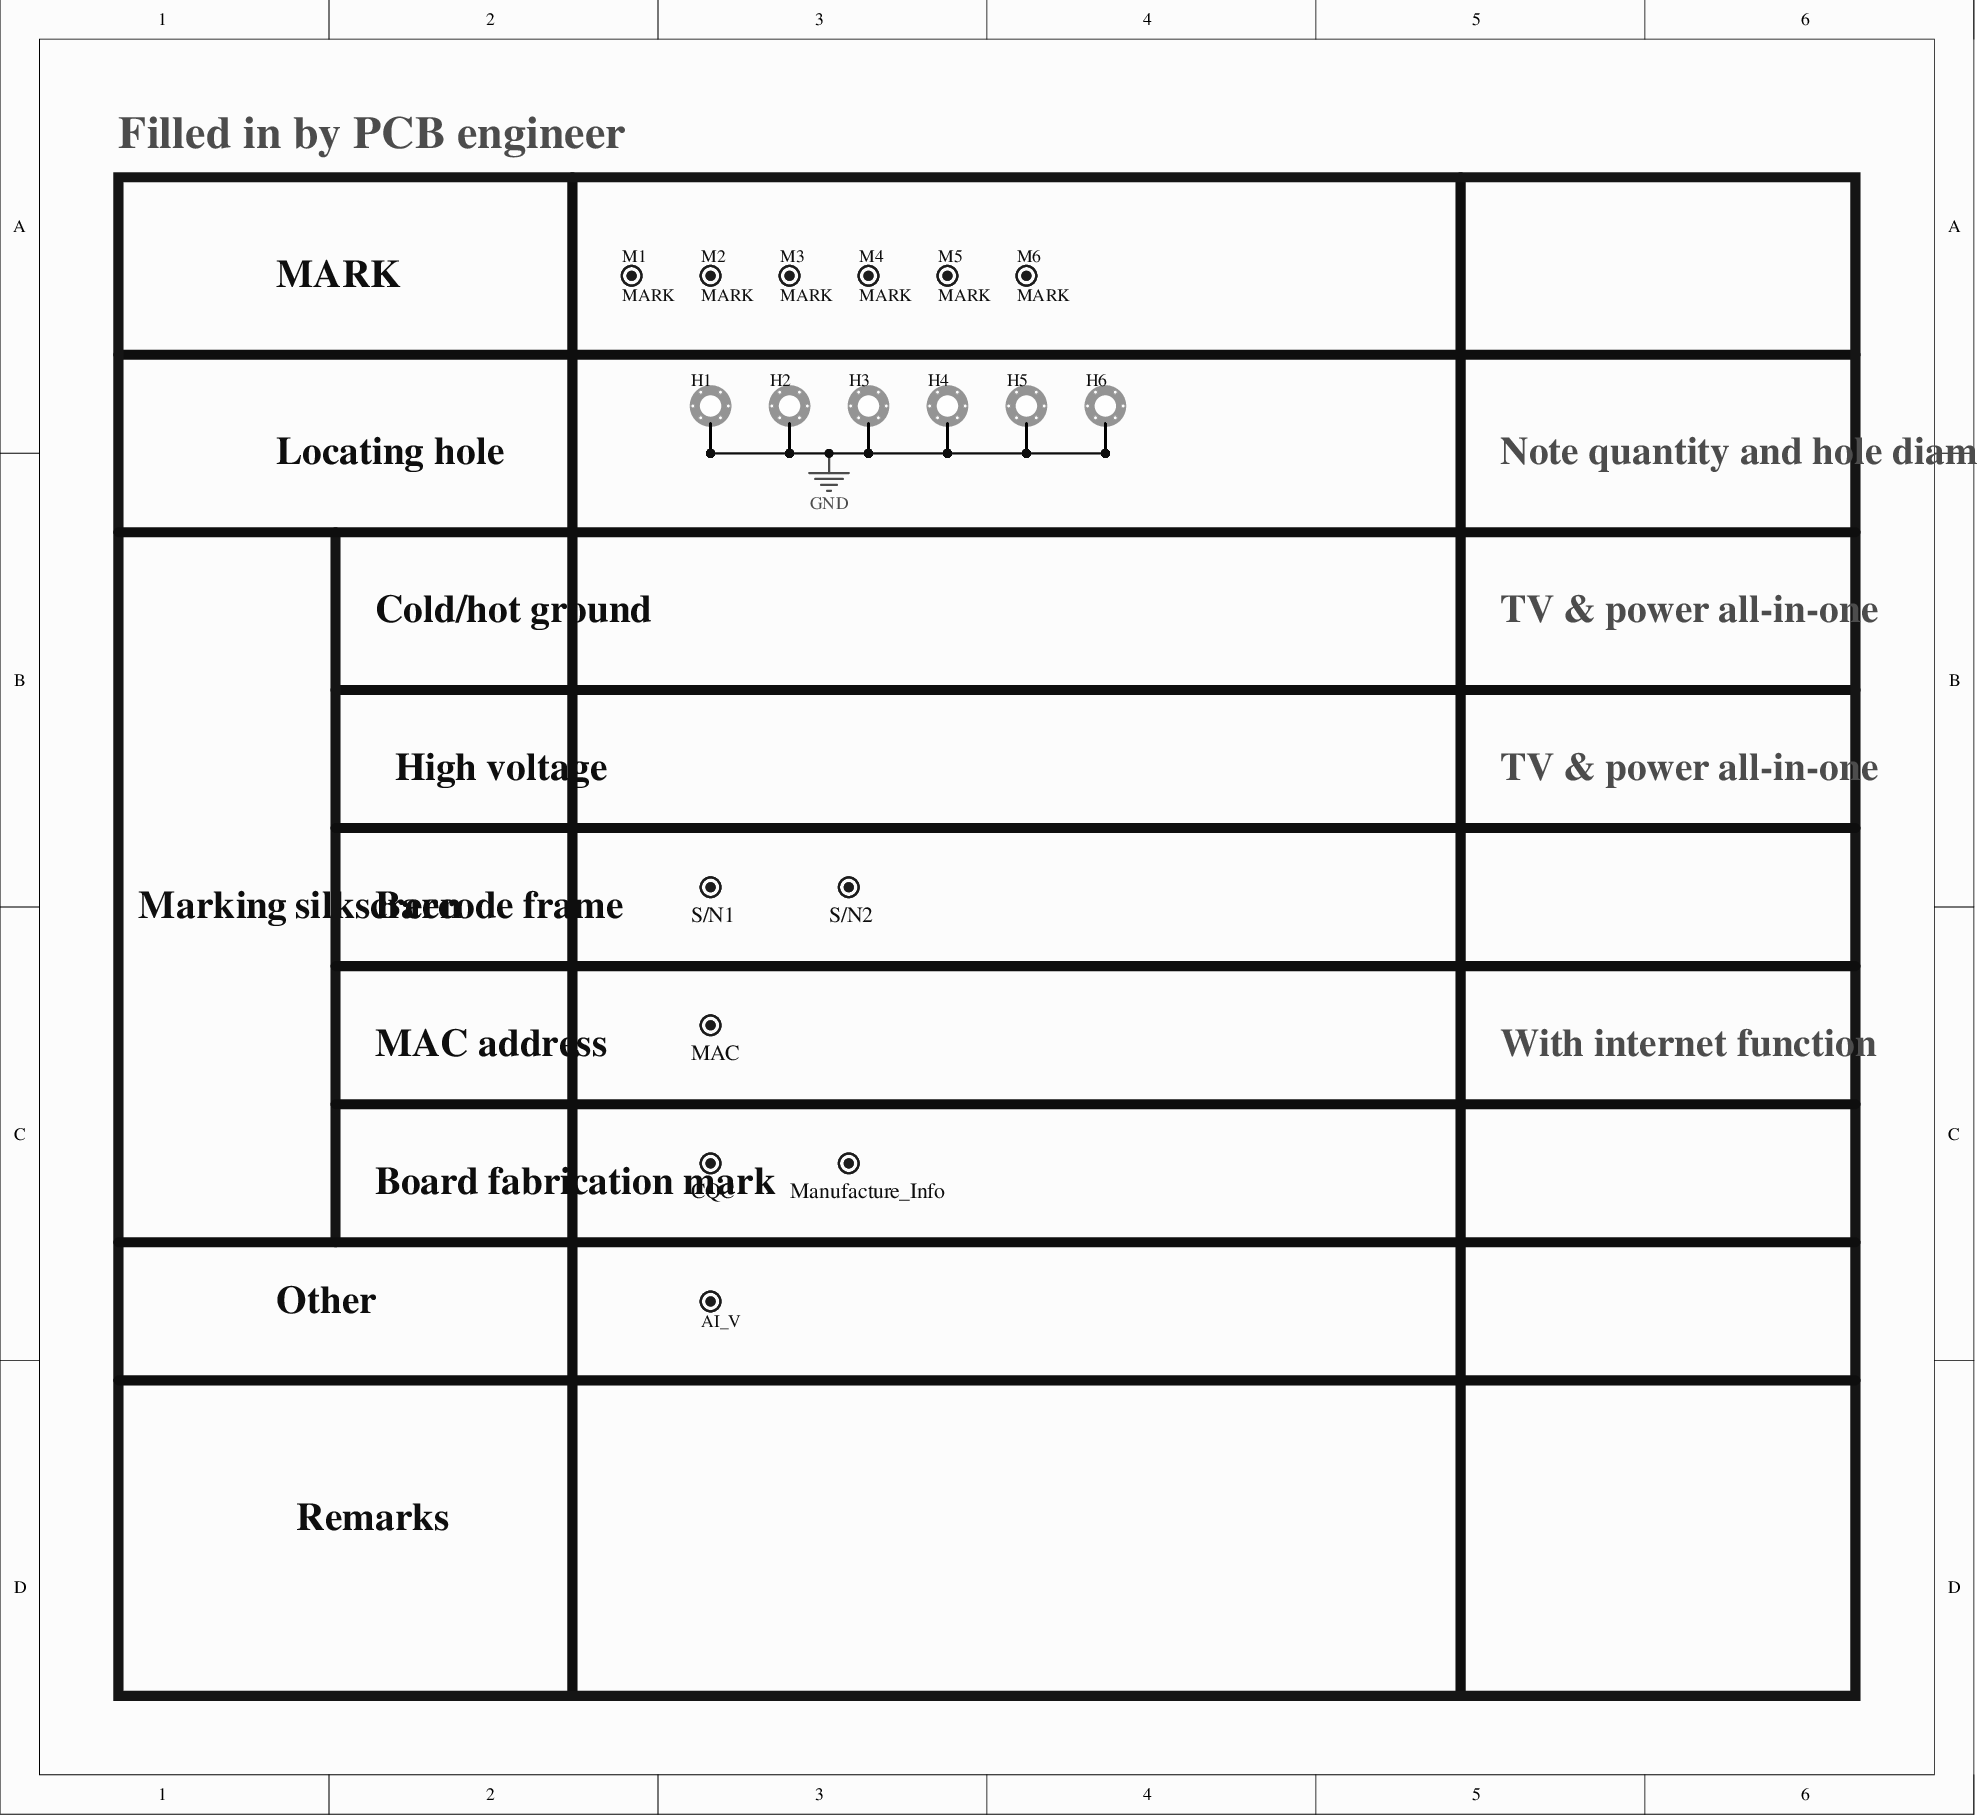
[diagram p0: MISC86290-2.SchDoc]
# Altium project MISC86290.PrjPcb (part 1 of 13)
17 sheets, 1041 parts. Net scope: global (net labels, ports and power ports of the same name join across sheets).
Board file: MISC86290.PcbDoc
Sheets:
  MISC86290-2.SchDoc
  MISC86290-3.SchDoc
  MISC86290-5.SchDoc
  MISC86290-6.SchDoc
  MISC86290-7.SchDoc
  MISC86290-8.SchDoc
  MISC86290-9.SchDoc
  MISC86290-10.SchDoc
  MISC86290-11.SchDoc
  MISC86290-12.SchDoc
  MISC86290-13.SchDoc
  MISC86290-14.SchDoc
  MISC86290-15.SchDoc
  MISC86290-16.SchDoc
  MISC86290-17.SchDoc
  MISC86290-18.SchDoc
  MISC86290-19.SchDoc

## Sheet MISC86290-2.SchDoc
size 254 x 233 mm

### Parts
AI_V  AI_GRIPPER_V  [AI_GRIPPER_V]  (value not drawn)
CQC  CQC  [CQC]
H1  Location hole  [ASSE3.5C-3]  (value not drawn)
H2  Location hole  [ASSE3.5C-3]  (value not drawn)
H3  Location hole  [ASSE3.5C-3]  (value not drawn)
H4  Location hole  [ASSE3.5C-3]  (value not drawn)
H5  Location hole  [ASSE3.5C-3]  (value not drawn)
H6  Location hole  [ASSE5.0C-3]  (value not drawn)
M1  MARK  [MARK]
M2  MARK  [MARK]
M3  MARK  [MARK]
M4  MARK  [MARK]
M5  MARK  [MARK]
M6  MARK  [MARK]
MAC  MAC  [Barcode]  (value not drawn)
Manufacture_Info  Manufacture_Info  [Manufacture_Info]
S/N1  Barcode  [Barcode]  (value not drawn)
S/N2  Barcode  [Barcode]  (value not drawn)

### Nets
GND: H1.1 H1.2 H1.3 H1.4 H1.5 H1.6 H2.1 H2.2 H2.3 H2.4 H2.5 H2.6 H3.1 H3.2 H3.3 H3.4 H3.5 H3.6 H4.1 H4.2 H4.3 H4.4 H4.5 H4.6 H5.1 H5.2 H5.3 H5.4 H5.5 H5.6 H6.1 H6.2 H6.3 H6.4 H6.5 H6.6

### Notes on the sheet
- Filled in by PCB engineer
- MARK
- Locating hole
- Note quantity and hole diameter
- Cold/hot ground
- TV & power all-in-one
- High voltage
- Marking silkscreen
- Barcode frame
- MAC address
- With internet function
- (near CQC) Board fabrication mark
- Other
- Remarks

### Library data of the parts
H1-H6 = Location hole-D
M1-M6 = MARK-D
MAC = Barcode

## Sheet MISC86290-3.SchDoc
size 254 x 322 mm
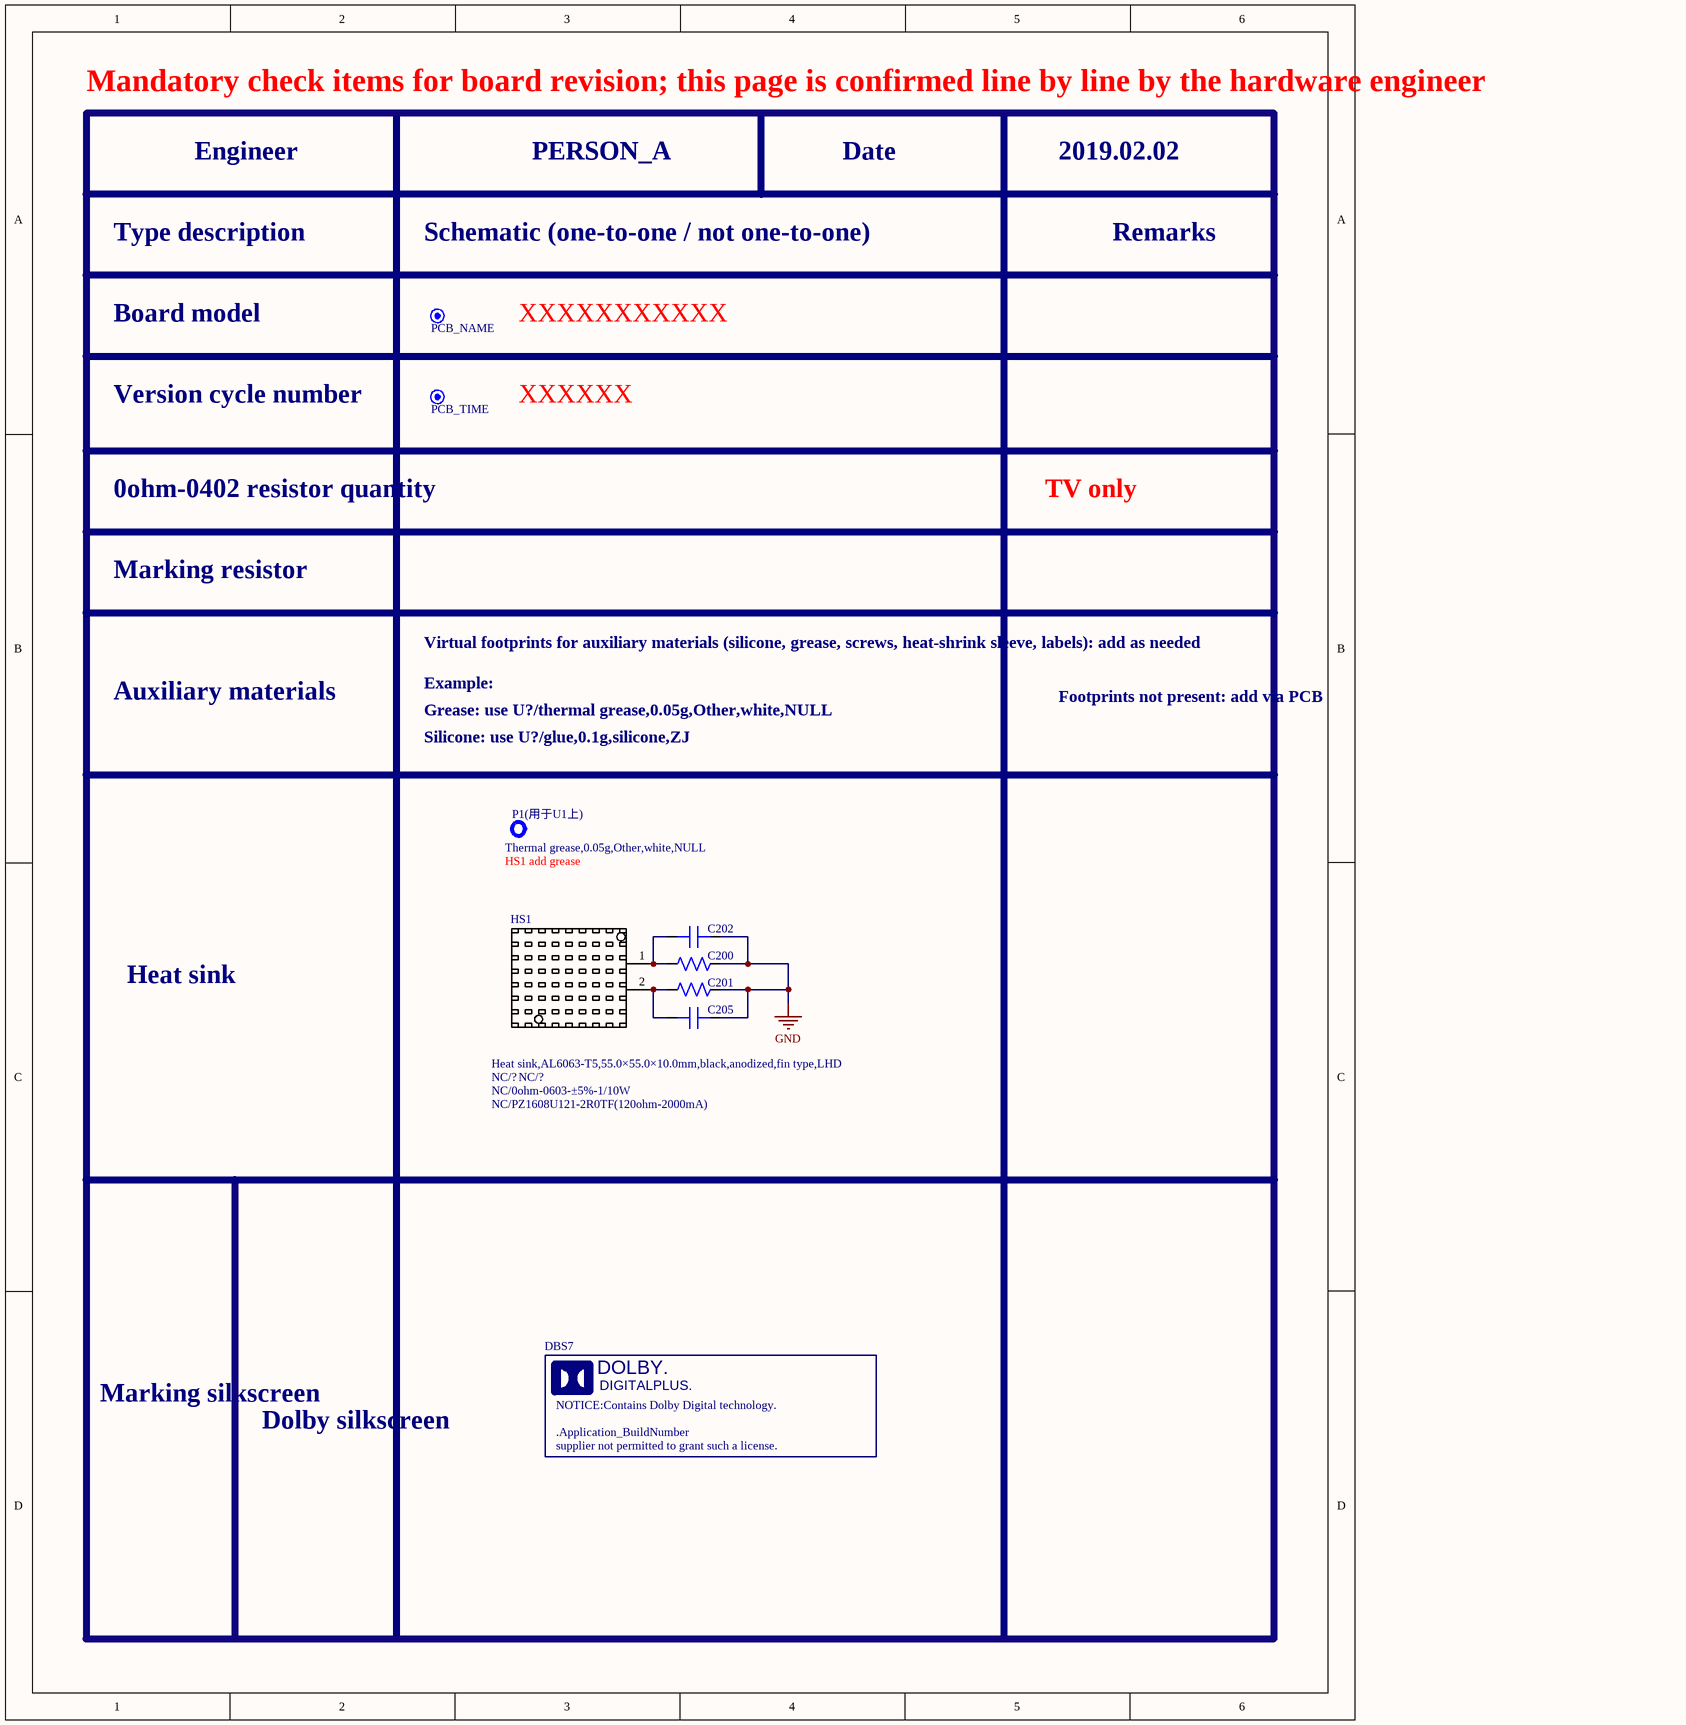
[diagram p1: MISC86290-3.SchDoc]

### Parts
C200  NC/0ohm-0603-±5%-1/10W  [R0603]
C201  NC/PZ1608U121-2R0TF(120ohm-2000mA)  [R0603]
C202  NC/?  [C0402]
C205  NC/?  [C0402]
DBS7  DOLBY PLUS  [DOLBY PLUS-SILK]  (value not drawn)
HS1  Heat sink,AL6063-T5,55.0×55.0×10.0mm,black,anodized,fin type,LHD  [HS(55*55*10)]
P1(用于U1上)  Thermal grease,0.05g,Other,white,NULL  [PCB_TIME]
XXXXXX  PCB_TIME  [PCB_TIME]
XXXXXXXXXXX  PCB_NAME  [PCB_NAME]

### Nets
GND: C200.2 C201.1 C202.1 C205.1
NetC200_1: C200.1 C202.2 HS1.1(GND)
NetC201_2: C201.2 C205.2 HS1.2(GND)

### Notes on the sheet
- Mandatory check items for board revision; this page is confirmed line by line by the hardware engineer
- Engineer
- PERSON_A
- Date
- 2019.02.02
- Type description
- Schematic (one-to-one / not one-to-one)
- Remarks
- Board model
- Version cycle number
- 0ohm-0402 resistor quantity
- TV only
- Marking resistor
- Virtual footprints for auxiliary materials (silicone, grease, screws, heat-shrink sleeve, labels): add as needed
- Auxiliary materials
- Example:
- Grease: use U?/thermal grease,0.05g,Other,white,NULL
- Footprints not present: add via PCB
- Silicone: use U?/glue,0.1g,silicone,ZJ
- (near P1(用于U1上)) HS1 add grease
- Heat sink
- Marking silkscreen
- Dolby silkscreen

### Library data of the parts
C200 C201 = 0ohm-0603-±5%-1/10W-D
C202 C205 = 1uF-0402-X5R-±20%-6.3V-D
HS1 = 004.040.0000611-HS: Heat sink,aluminium alloy,55.0×55.0×10.0mm,black,anodized,THD-HS
P1(用于U1上) = 0.05g-导热硅脂: Thermal grease